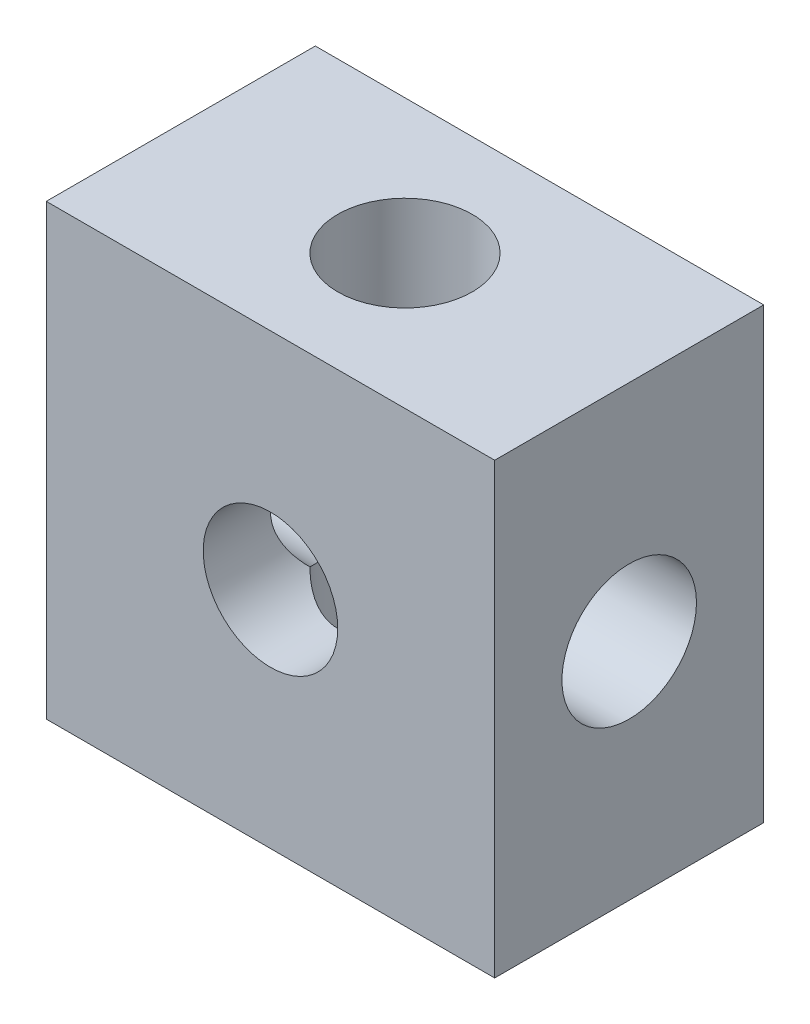
SolidWorks part; units mm, degrees
material "6061 合金"
ref_plane "前视基准面" through (0, 0, 0) normal (0, 0, 1) x (1, 0, 0)
ref_plane "上视基准面" through (0, 0, 0) normal (0, 1, 0) x (1, 0, 0)
ref_plane "右视基准面" through (0, 0, 0) normal (1, 0, 0) x (0, 0, -1)
other "Configuration Table"
sketch "草图1" plane through (0, 0, 0) normal (0, 1, 0) x (1, 0, 0)
  line L1 (0, 0) -> (10, 0)
  line L2 (0, 0) -> (0, 6)
  line L3 (0, 6) -> (10, 6)
  line L4 (10, 0) -> (10, 6)
  dimension "D1" = 6
  dimension "D2" = 10
extrude "凸台-拉伸1" add sketch "草图1" along normal blind 10
sketch "草图2" plane through (0, 0, 0) normal (0, 0, 1) x (1, 0, 0)
  line L0 (5, 10) -> (5, 0) construction
  line L1 (0, 10) -> (10, 10) construction
  line L2 (0, 0) -> (10, 0) construction
  circle A0 centre (5, 5) radius 1.5
  dimension "D1" = 3
sketch "草图3" plane through (10, 0, 0) normal (1, 0, 0) x (0, 0, -1)
  line L0 (3, 10) -> (3, 0) construction
  line L1 (0, 10) -> (6, 10) construction
  line L2 (0, 0) -> (6, 0) construction
  circle A0 centre (3, 5) radius 1.5
  dimension "D1" = 3
sketch "草图4" plane through (0, 10, 0) normal (0, 1, 0) x (1, 0, 0)
  line L0 (0, 3) -> (10, 3) construction
  line L1 (0, 6) -> (0, 0) construction
  line L2 (10, 1.5) -> (10, 4.5) construction
  circle A0 centre (5, 3) radius 1.5
  dimension "D1" = 3
extrude "切除-拉伸1" cut sketch "草图2" against normal through all
extrude "切除-拉伸2" cut sketch "草图4" against normal through all
extrude "切除-拉伸3" cut sketch "草图3" against normal through all
